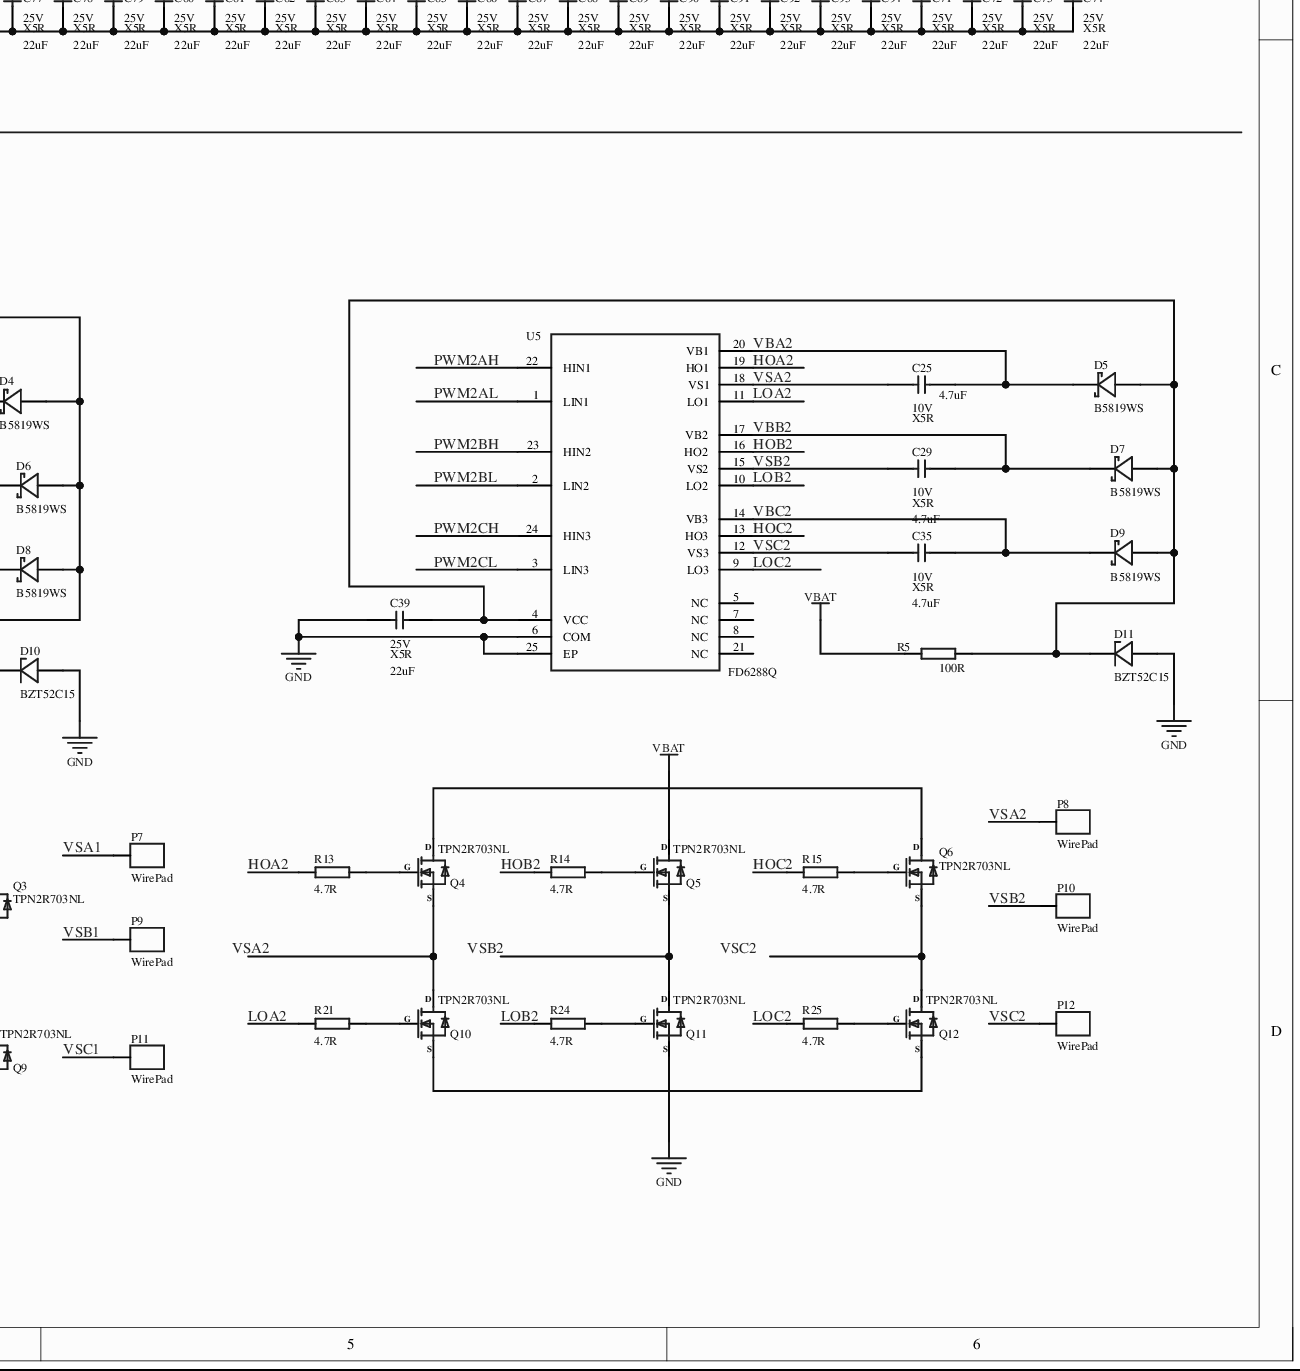
[diagram p0: MISC49862-3.schdoc, bottom right]
# Altium project MISC49862-2.PrjPcb (part 2 of 4)

## Sheet MISC49862-3.schdoc (continued)
### Library data of the parts
C1 = =Value +' '+ Voltage + ' ' + Type: SMD ceramic capacitor; MLCC; 0402(1005);; Device: 4.7uF 10V X5R; Symbol: 4.7uF 0402 10V X5R; Origin Footprint 2: CAPC1005[0402]-L; Origin Footprint 3: CAPC1005[0402]-M; Origin Footprint 4: CAPC1005[0402]-N; Origin Footprint 5: CAPC1005[0402]S-L; Origin Footprint 6: CAPC1005[0402]S-M; UniqueId: b4693cfd16d534cd; AddInBom: yes; Origin Footprint 1: CAPC1005[0402]S-N; Design Item ID: 4.7uF 0402 10V X5R; Library Name: Brushless driver-CYT2BL3-FD6288-FOC-LiteDual; Revision: V1.0; FootprintName: CAPC1005[0402]S-N; ConvertToPcb: yes
C2 = =Value +' '+ Voltage + ' ' + Type: SMD ceramic capacitor; MLCC; 0402(1005);; Device: 100nF 16V X7R; Symbol: 100nF 0402 16V X7R; Origin Footprint 2: CAPC1005[0402]-L; Origin Footprint 3: CAPC1005[0402]-M; Origin Footprint 4: CAPC1005[0402]-N; Origin Footprint 5: CAPC1005[0402]S-L; Origin Footprint 6: CAPC1005[0402]S-M; UniqueId: a2c5d49bc5dde298; AddInBom: yes; Origin Footprint 1: CAPC1005[0402]S-N; Design Item ID: 100nF 0402 16V X7R; Library Name: Brushless driver-CYT2BL3-FD6288-FOC-LiteDual; Revision: V1.0; FootprintName: CAPC1005[0402]S-N; ConvertToPcb: yes
C3 = =Value +' '+ Voltage + ' ' + Type: SMD ceramic capacitor; MLCC; 0402(1005);; Device: 4.7uF 10V X5R; Symbol: 4.7uF 0402 10V X5R; Origin Footprint 2: CAPC1005[0402]-L; Origin Footprint 3: CAPC1005[0402]-M; Origin Footprint 4: CAPC1005[0402]-N; Origin Footprint 5: CAPC1005[0402]S-L; Origin Footprint 6: CAPC1005[0402]S-M; UniqueId: cc82bf2c2e22e605; AddInBom: yes; Origin Footprint 1: CAPC1005[0402]S-N; Design Item ID: 4.7uF 0402 10V X5R; Library Name: Brushless driver-CYT2BL3-FD6288-FOC-LiteDual; Revision: V1.0; FootprintName: CAPC1005[0402]S-N; ConvertToPcb: yes
C4 = =Value +' '+ Voltage + ' ' + Type: SMD ceramic capacitor; MLCC; 0402(1005);; Device: 100nF 16V X7R; Symbol: 100nF 0402 16V X7R; Origin Footprint 2: CAPC1005[0402]-L; Origin Footprint 3: CAPC1005[0402]-M; Origin Footprint 4: CAPC1005[0402]-N; Origin Footprint 5: CAPC1005[0402]S-L; Origin Footprint 6: CAPC1005[0402]S-M; UniqueId: 3a68d3ddabf48558; AddInBom: yes; Origin Footprint 1: CAPC1005[0402]S-N; Design Item ID: 100nF 0402 16V X7R; Library Name: Brushless driver-CYT2BL3-FD6288-FOC-LiteDual; Revision: V1.0; FootprintName: CAPC1005[0402]S-N; ConvertToPcb: yes
C5 = =Value +' '+ Voltage + ' ' + Type: SMD ceramic capacitor; MLCC; 0402(1005);; Device: 2.2uF 10V X5R; Symbol: 2.2uF 0402 10V X5R; Origin Footprint 2: CAPC1005[0402]-L; Origin Footprint 3: CAPC1005[0402]-M; Origin Footprint 4: CAPC1005[0402]-N; Origin Footprint 5: CAPC1005[0402]S-L; Origin Footprint 6: CAPC1005[0402]S-M; UniqueId: ddba3c46cf8b8e66; AddInBom: yes; Origin Footprint 1: CAPC1005[0402]S-N; Design Item ID: 2.2uF 0402 10V X5R; Library Name: Brushless driver-CYT2BL3-FD6288-FOC-LiteDual; Revision: V1.0; FootprintName: CAPC1005[0402]S-N; ConvertToPcb: yes
C6 = =Value +' '+ Voltage + ' ' + Type: SMD ceramic capacitor; MLCC; 0402(1005);; Device: 100nF 16V X7R; Symbol: 100nF 0402 16V X7R; Origin Footprint 2: CAPC1005[0402]-L; Origin Footprint 3: CAPC1005[0402]-M; Origin Footprint 4: CAPC1005[0402]-N; Origin Footprint 5: CAPC1005[0402]S-L; Origin Footprint 6: CAPC1005[0402]S-M; UniqueId: ab4a8fe24fad9fe4; AddInBom: yes; Origin Footprint 1: CAPC1005[0402]S-N; Design Item ID: 100nF 0402 16V X7R; Library Name: Brushless driver-CYT2BL3-FD6288-FOC-LiteDual; Revision: V1.0; FootprintName: CAPC1005[0402]S-N; ConvertToPcb: yes
C7 = =Value +' '+ Voltage + ' ' + Type: SMD ceramic capacitor; MLCC; 0402(1005);; Device: 100nF 16V X7R; Symbol: 100nF 0402 16V X7R; Origin Footprint 2: CAPC1005[0402]-L; Origin Footprint 3: CAPC1005[0402]-M; Origin Footprint 4: CAPC1005[0402]-N; Origin Footprint 5: CAPC1005[0402]S-L; Origin Footprint 6: CAPC1005[0402]S-M; UniqueId: 48d2dd422533522c; AddInBom: yes; Origin Footprint 1: CAPC1005[0402]S-N; Design Item ID: 100nF 0402 16V X7R; Library Name: Brushless driver-CYT2BL3-FD6288-FOC-LiteDual; Revision: V1.0; FootprintName: CAPC1005[0402]S-N; ConvertToPcb: yes
C8 = =Value +' '+ Voltage + ' ' + Type: SMD ceramic capacitor; MLCC; 0402(1005);; Device: 4.7uF 10V X5R; Symbol: 4.7uF 0402 10V X5R; Origin Footprint 2: CAPC1005[0402]-L; Origin Footprint 3: CAPC1005[0402]-M; Origin Footprint 4: CAPC1005[0402]-N; Origin Footprint 5: CAPC1005[0402]S-L; Origin Footprint 6: CAPC1005[0402]S-M; UniqueId: 80f3708378e3d903; AddInBom: yes; Origin Footprint 1: CAPC1005[0402]S-N; Design Item ID: 4.7uF 0402 10V X5R; Library Name: Brushless driver-CYT2BL3-FD6288-FOC-LiteDual; Revision: V1.0; FootprintName: CAPC1005[0402]S-N; ConvertToPcb: yes
C9 = =Value +' '+ Voltage + ' ' + Type: SMD ceramic capacitor; MLCC; 0402(1005);; Device: 4.7uF 10V X5R; Symbol: 4.7uF 0402 10V X5R; Origin Footprint 2: CAPC1005[0402]-L; Origin Footprint 3: CAPC1005[0402]-M; Origin Footprint 4: CAPC1005[0402]-N; Origin Footprint 5: CAPC1005[0402]S-L; Origin Footprint 6: CAPC1005[0402]S-M; UniqueId: 7ddfd2f632a8b17d; AddInBom: yes; Origin Footprint 1: CAPC1005[0402]S-N; Design Item ID: 4.7uF 0402 10V X5R; Library Name: Brushless driver-CYT2BL3-FD6288-FOC-LiteDual; Revision: V1.0; FootprintName: CAPC1005[0402]S-N; ConvertToPcb: yes
C10 = =Value +' '+ Voltage + ' ' + Type: SMD ceramic capacitor; MLCC; 0402(1005);; Device: 100nF 16V X7R; Symbol: 100nF 0402 16V X7R; Origin Footprint 2: CAPC1005[0402]-L; Origin Footprint 3: CAPC1005[0402]-M; Origin Footprint 4: CAPC1005[0402]-N; Origin Footprint 5: CAPC1005[0402]S-L; Origin Footprint 6: CAPC1005[0402]S-M; UniqueId: 3e75135af30e0f04; AddInBom: yes; Origin Footprint 1: CAPC1005[0402]S-N; Design Item ID: 100nF 0402 16V X7R; Library Name: Brushless driver-CYT2BL3-FD6288-FOC-LiteDual; Revision: V1.0; FootprintName: CAPC1005[0402]S-N; ConvertToPcb: yes
C11 = =Value +' '+ Voltage + ' ' + Type: SMD ceramic capacitor; MLCC; 0402(1005);; Device: 100nF 16V X7R; Symbol: 100nF 0402 16V X7R; Origin Footprint 2: CAPC1005[0402]-L; Origin Footprint 3: CAPC1005[0402]-M; Origin Footprint 4: CAPC1005[0402]-N; Origin Footprint 5: CAPC1005[0402]S-L; Origin Footprint 6: CAPC1005[0402]S-M; UniqueId: 20764de07767b3a1; AddInBom: yes; Origin Footprint 1: CAPC1005[0402]S-N; Design Item ID: 100nF 0402 16V X7R; Library Name: Brushless driver-CYT2BL3-FD6288-FOC-LiteDual; Revision: V1.0; FootprintName: CAPC1005[0402]S-N; ConvertToPcb: yes
C12 = =Value +' '+ Voltage + ' ' + Type: SMD ceramic capacitor; MLCC; 0402(1005);; Device: 4.7uF 10V X5R; Symbol: 4.7uF 0402 10V X5R; Origin Footprint 2: CAPC1005[0402]-L; Origin Footprint 3: CAPC1005[0402]-M; Origin Footprint 4: CAPC1005[0402]-N; Origin Footprint 5: CAPC1005[0402]S-L; Origin Footprint 6: CAPC1005[0402]S-M; UniqueId: 26a39bcafcc8ce7c; AddInBom: yes; Origin Footprint 1: CAPC1005[0402]S-N; Design Item ID: 4.7uF 0402 10V X5R; Library Name: Brushless driver-CYT2BL3-FD6288-FOC-LiteDual; Revision: V1.0; FootprintName: CAPC1005[0402]S-N; ConvertToPcb: yes
C13 = =Value +' '+ Voltage + ' ' + Type: SMD ceramic capacitor; MLCC; 0402(1005);; Device: 100nF 16V X7R; Symbol: 100nF 0402 16V X7R; Origin Footprint 2: CAPC1005[0402]-L; Origin Footprint 3: CAPC1005[0402]-M; Origin Footprint 4: CAPC1005[0402]-N; Origin Footprint 5: CAPC1005[0402]S-L; Origin Footprint 6: CAPC1005[0402]S-M; UniqueId: e7ba3aba9f9889c8; AddInBom: yes; Origin Footprint 1: CAPC1005[0402]S-N; Design Item ID: 100nF 0402 16V X7R; Library Name: Brushless driver-CYT2BL3-FD6288-FOC-LiteDual; Revision: V1.0; FootprintName: CAPC1005[0402]S-N; ConvertToPcb: yes
C14 = =Value +' '+ Voltage + ' ' + Type: SMD ceramic capacitor; MLCC; 0402(1005);; Device: 4.7uF 10V X5R; Symbol: 4.7uF 0402 10V X5R; Origin Footprint 2: CAPC1005[0402]-L; Origin Footprint 3: CAPC1005[0402]-M; Origin Footprint 4: CAPC1005[0402]-N; Origin Footprint 5: CAPC1005[0402]S-L; Origin Footprint 6: CAPC1005[0402]S-M; UniqueId: 00361082df9d4549; AddInBom: yes; Origin Footprint 1: CAPC1005[0402]S-N; Design Item ID: 4.7uF 0402 10V X5R; Library Name: Brushless driver-CYT2BL3-FD6288-FOC-LiteDual; Revision: V1.0; FootprintName: CAPC1005[0402]S-N; ConvertToPcb: yes
C15 = =Value +' '+ Voltage + ' ' + Type: SMD ceramic capacitor; MLCC; 0402(1005);; Device: 10pF 50V C0G; Symbol: 10pF 0402 50V C0G; Origin Footprint 2: CAPC1005[0402]-L; Origin Footprint 3: CAPC1005[0402]-M; Origin Footprint 4: CAPC1005[0402]-N; Origin Footprint 5: CAPC1005[0402]S-L; Origin Footprint 6: CAPC1005[0402]S-M; UniqueId: 86bb77bda672094d; AddInBom: yes; Origin Footprint 1: CAPC1005[0402]S-N; Design Item ID: 10pF 0402 50V C0G; Library Name: Brushless driver-CYT2BL3-FD6288-FOC-LiteDual; Revision: V1.0; FootprintName: CAPC1005[0402]S-N; ConvertToPcb: yes
C16 = =Value +' '+ Voltage + ' ' + Type: SMD ceramic capacitor; MLCC; 0402(1005);; Device: 10pF 50V C0G; Symbol: 10pF 0402 50V C0G; Origin Footprint 2: CAPC1005[0402]-L; Origin Footprint 3: CAPC1005[0402]-M; Origin Footprint 4: CAPC1005[0402]-N; Origin Footprint 5: CAPC1005[0402]S-L; Origin Footprint 6: CAPC1005[0402]S-M; UniqueId: c8e923f96b539988; AddInBom: yes; Origin Footprint 1: CAPC1005[0402]S-N; Design Item ID: 10pF 0402 50V C0G; Library Name: Brushless driver-CYT2BL3-FD6288-FOC-LiteDual; Revision: V1.0; FootprintName: CAPC1005[0402]S-N; ConvertToPcb: yes
C17 = =Value +' '+ Voltage + ' ' + Type: SMD ceramic capacitor; MLCC; 0402(1005);; Device: 100nF 16V X7R; Symbol: 100nF 0402 16V X7R; Origin Footprint 2: CAPC1005[0402]-L; Origin Footprint 3: CAPC1005[0402]-M; Origin Footprint 4: CAPC1005[0402]-N; Origin Footprint 5: CAPC1005[0402]S-L; Origin Footprint 6: CAPC1005[0402]S-M; UniqueId: 48700c84863a802e; AddInBom: yes; Origin Footprint 1: CAPC1005[0402]S-N; Design Item ID: 100nF 0402 16V X7R; Library Name: Brushless driver-CYT2BL3-FD6288-FOC-LiteDual; Revision: V1.0; FootprintName: CAPC1005[0402]S-N; ConvertToPcb: yes
C18 = =Value +' '+ Voltage + ' ' + Type: SMD ceramic capacitor; MLCC; 0402(1005);; Device: 4.7uF 10V X5R; Symbol: 4.7uF 0402 10V X5R; Origin Footprint 2: CAPC1005[0402]-L; Origin Footprint 3: CAPC1005[0402]-M; Origin Footprint 4: CAPC1005[0402]-N; Origin Footprint 5: CAPC1005[0402]S-L; Origin Footprint 6: CAPC1005[0402]S-M; UniqueId: d9d0285421fe3ef0; AddInBom: yes; Origin Footprint 1: CAPC1005[0402]S-N; Design Item ID: 4.7uF 0402 10V X5R; Library Name: SEEKFREE_Capacitor; Revision: V1.0; FootprintName: CAPC1005[0402]S-N; ConvertToPcb: yes
C19 = =Value +' '+ Voltage + ' ' + Type: SMD ceramic capacitor; MLCC; 0805(2012);; Device: 22uF 25V X5R; Symbol: 22uF 0805 25V X5R; Origin Footprint 2: CAPC2012[0805]; Origin Footprint 3: CAPC2012[0805]S-L; Origin Footprint 4: CAPC2012[0805]S-M; UniqueId: 9b75bd895f0e39d2; AddInBom: yes; Origin Footprint 1: CAPC2012[0805]S-N; Design Item ID: 22uF 0805 25V X5R; Library Name: SEEKFREE_Capacitor; Revision: V1.0; FootprintName: CAPC2012[0805]S-N; ConvertToPcb: yes
C20 = =Value +' '+ Voltage + ' ' + Type: SMD ceramic capacitor; MLCC; 0805(2012);; Device: 22uF 25V X5R; Symbol: 22uF 0805 25V X5R; Origin Footprint 2: CAPC2012[0805]; Origin Footprint 3: CAPC2012[0805]S-L; Origin Footprint 4: CAPC2012[0805]S-M; UniqueId: 97d7532320e593d5; AddInBom: yes; Origin Footprint 1: CAPC2012[0805]S-N; Design Item ID: 22uF 0805 25V X5R; Library Name: SEEKFREE_Capacitor; Revision: V1.0; FootprintName: CAPC2012[0805]S-N; ConvertToPcb: yes
C21 = =Value +' '+ Voltage + ' ' + Type: SMD ceramic capacitor; MLCC; 0402(1005);; Device: 100nF 16V X7R; Symbol: 100nF 0402 16V X7R; Origin Footprint 2: CAPC1005[0402]-L; Origin Footprint 3: CAPC1005[0402]-M; Origin Footprint 4: CAPC1005[0402]-N; Origin Footprint 5: CAPC1005[0402]S-L; Origin Footprint 6: CAPC1005[0402]S-M; UniqueId: 0259cc883dd91c7a; AddInBom: yes; Origin Footprint 1: CAPC1005[0402]S-N; Design Item ID: 100nF 0402 16V X7R; Library Name: Brushless driver-CYT2BL3-FD6288-FOC-LiteDual; Revision: V1.0; FootprintName: CAPC1005[0402]S-N; ConvertToPcb: yes
C22 = =Value +' '+ Voltage + ' ' + Type: SMD ceramic capacitor; MLCC; 0402(1005);; Device: 220pF 50V X7R; Symbol: 220pF 0402 50V X7R; Origin Footprint 2: CAPC1005[0402]-L; Origin Footprint 3: CAPC1005[0402]-M; Origin Footprint 4: CAPC1005[0402]-N; Origin Footprint 5: CAPC1005[0402]S-L; Origin Footprint 6: CAPC1005[0402]S-M; UniqueId: 7f35450ac3171d20; AddInBom: yes; Origin Footprint 1: CAPC1005[0402]S-N; Design Item ID: 220pF 0402 50V X7R; Library Name: Brushless driver-CYT2BL3-FD6288-FOC-LiteDual; Revision: V1.0; FootprintName: CAPC1005[0402]S-N; ConvertToPcb: yes
C23 = =Value +' '+ Voltage + ' ' + Type: SMD ceramic capacitor; MLCC; 0805(2012);; Device: 22uF 25V X5R; Symbol: 22uF 0805 25V X5R; Origin Footprint 2: CAPC2012[0805]; Origin Footprint 3: CAPC2012[0805]S-L; Origin Footprint 4: CAPC2012[0805]S-M; UniqueId: 8bc5c1e1749a19fa; AddInBom: yes; Origin Footprint 1: CAPC2012[0805]S-N; Design Item ID: 22uF 0805 25V X5R; Library Name: Brushless driver-CYT2BL3-FD6288-FOC-LiteDual; Revision: V1.0; FootprintName: CAPC2012[0805]S-N; ConvertToPcb: yes
C24 = =Value +' '+ Voltage + ' ' + Type: SMD ceramic capacitor; MLCC; 0402(1005);; Device: 100nF 16V X7R; Symbol: 100nF 0402 16V X7R; Origin Footprint 2: CAPC1005[0402]-L; Origin Footprint 3: CAPC1005[0402]-M; Origin Footprint 4: CAPC1005[0402]-N; Origin Footprint 5: CAPC1005[0402]S-L; Origin Footprint 6: CAPC1005[0402]S-M; UniqueId: 7c674fedd66d7165; AddInBom: yes; Origin Footprint 1: CAPC1005[0402]S-N; Design Item ID: 100nF 0402 16V X7R; Library Name: Brushless driver-CYT2BL3-FD6288-FOC-LiteDual; Revision: V1.0; FootprintName: CAPC1005[0402]S-N; ConvertToPcb: yes
C25 = =Value +' '+ Voltage + ' ' + Type: SMD ceramic capacitor; MLCC; 0402(1005);; Device: 4.7uF 10V X5R; Symbol: 4.7uF 0402 10V X5R; Origin Footprint 2: CAPC1005[0402]-L; Origin Footprint 3: CAPC1005[0402]-M; Origin Footprint 4: CAPC1005[0402]-N; Origin Footprint 5: CAPC1005[0402]S-L; Origin Footprint 6: CAPC1005[0402]S-M; UniqueId: d99985aa138ce050; AddInBom: yes; Origin Footprint 1: CAPC1005[0402]S-N; Design Item ID: 4.7uF 0402 10V X5R; Library Name: SEEKFREE_Capacitor; Revision: V1.0; FootprintName: CAPC1005[0402]S-N; ConvertToPcb: yes
C26 = =Value +' '+ Voltage + ' ' + Type: SMD ceramic capacitor; MLCC; 0805(2012);; Device: 22uF 25V X5R; Symbol: 22uF 0805 25V X5R; Origin Footprint 2: CAPC2012[0805]; Origin Footprint 3: CAPC2012[0805]S-L; Origin Footprint 4: CAPC2012[0805]S-M; UniqueId: 5bc8fc857418e778; AddInBom: yes; Origin Footprint 1: CAPC2012[0805]S-N; Design Item ID: 22uF 0805 25V X5R; Library Name: Brushless driver-CYT2BL3-FD6288-FOC-LiteDual; Revision: V1.0; FootprintName: CAPC2012[0805]S-N; ConvertToPcb: yes
C27 = =Value +' '+ Voltage + ' ' + Type: SMD ceramic capacitor; MLCC; 0402(1005);; Device: 100nF 16V X7R; Symbol: 100nF 0402 16V X7R; Origin Footprint 2: CAPC1005[0402]-L; Origin Footprint 3: CAPC1005[0402]-M; Origin Footprint 4: CAPC1005[0402]-N; Origin Footprint 5: CAPC1005[0402]S-L; Origin Footprint 6: CAPC1005[0402]S-M; UniqueId: a26eb100929f0697; AddInBom: yes; Origin Footprint 1: CAPC1005[0402]S-N; Design Item ID: 100nF 0402 16V X7R; Library Name: Brushless driver-CYT2BL3-FD6288-FOC-LiteDual; Revision: V1.0; FootprintName: CAPC1005[0402]S-N; ConvertToPcb: yes
C28 = =Value +' '+ Voltage + ' ' + Type: SMD ceramic capacitor; MLCC; 0402(1005);; Device: 4.7uF 10V X5R; Symbol: 4.7uF 0402 10V X5R; Origin Footprint 2: CAPC1005[0402]-L; Origin Footprint 3: CAPC1005[0402]-M; Origin Footprint 4: CAPC1005[0402]-N; Origin Footprint 5: CAPC1005[0402]S-L; Origin Footprint 6: CAPC1005[0402]S-M; UniqueId: e3aeb17489c0ab5d; AddInBom: yes; Origin Footprint 1: CAPC1005[0402]S-N; Design Item ID: 4.7uF 0402 10V X5R; Library Name: SEEKFREE_Capacitor; Revision: V1.0; FootprintName: CAPC1005[0402]S-N; ConvertToPcb: yes
C29 = =Value +' '+ Voltage + ' ' + Type: SMD ceramic capacitor; MLCC; 0402(1005);; Device: 4.7uF 10V X5R; Symbol: 4.7uF 0402 10V X5R; Origin Footprint 2: CAPC1005[0402]-L; Origin Footprint 3: CAPC1005[0402]-M; Origin Footprint 4: CAPC1005[0402]-N; Origin Footprint 5: CAPC1005[0402]S-L; Origin Footprint 6: CAPC1005[0402]S-M; UniqueId: 5bfcee5f0e3d202c; AddInBom: yes; Origin Footprint 1: CAPC1005[0402]S-N; Design Item ID: 4.7uF 0402 10V X5R; Library Name: SEEKFREE_Capacitor; Revision: V1.0; FootprintName: CAPC1005[0402]S-N; ConvertToPcb: yes
C30 = =Value +' '+ Voltage + ' ' + Type: SMD ceramic capacitor; MLCC; 0402(1005);; Device: 4.7uF 10V X5R; Symbol: 4.7uF 0402 10V X5R; Origin Footprint 2: CAPC1005[0402]-L; Origin Footprint 3: CAPC1005[0402]-M; Origin Footprint 4: CAPC1005[0402]-N; Origin Footprint 5: CAPC1005[0402]S-L; Origin Footprint 6: CAPC1005[0402]S-M; UniqueId: a2ee6ceb65d30336; AddInBom: yes; Origin Footprint 1: CAPC1005[0402]S-N; Design Item ID: 4.7uF 0402 10V X5R; Library Name: SEEKFREE_Capacitor; Revision: V1.0; FootprintName: CAPC1005[0402]S-N; ConvertToPcb: yes
C31 = =Value +' '+ Voltage + ' ' + Type: SMD ceramic capacitor; MLCC; 0402(1005);; Device: 100nF 16V X7R; Symbol: 100nF 0402 16V X7R; Origin Footprint 2: CAPC1005[0402]-L; Origin Footprint 3: CAPC1005[0402]-M; Origin Footprint 4: CAPC1005[0402]-N; Origin Footprint 5: CAPC1005[0402]S-L; Origin Footprint 6: CAPC1005[0402]S-M; UniqueId: cc1d00c51cc12124; AddInBom: yes; Origin Footprint 1: CAPC1005[0402]S-N; Design Item ID: 100nF 0402 16V X7R; Library Name: Brushless driver-CYT2BL3-FD6288-FOC-LiteDual; Revision: V1.0; FootprintName: CAPC1005[0402]S-N; ConvertToPcb: yes
C32 = =Value +' '+ Voltage + ' ' + Type: SMD ceramic capacitor; MLCC; 0402(1005);; Device: 220pF 50V X7R; Symbol: 220pF 0402 50V X7R; Origin Footprint 2: CAPC1005[0402]-L; Origin Footprint 3: CAPC1005[0402]-M; Origin Footprint 4: CAPC1005[0402]-N; Origin Footprint 5: CAPC1005[0402]S-L; Origin Footprint 6: CAPC1005[0402]S-M; UniqueId: d2625f4b4bd439ef; AddInBom: yes; Origin Footprint 1: CAPC1005[0402]S-N; Design Item ID: 220pF 0402 50V X7R; Library Name: Brushless driver-CYT2BL3-FD6288-FOC-LiteDual; Revision: V1.0; FootprintName: CAPC1005[0402]S-N; ConvertToPcb: yes
C33 = =Value +' '+ Voltage + ' ' + Type: SMD ceramic capacitor; MLCC; 0805(2012);; Device: 22uF 25V X5R; Symbol: 22uF 0805 25V X5R; Origin Footprint 2: CAPC2012[0805]; Origin Footprint 3: CAPC2012[0805]S-L; Origin Footprint 4: CAPC2012[0805]S-M; UniqueId: deb55bbe20a101cf; AddInBom: yes; Origin Footprint 1: CAPC2012[0805]S-N; Design Item ID: 22uF 0805 25V X5R; Library Name: Brushless driver-CYT2BL3-FD6288-FOC-LiteDual; Revision: V1.0; FootprintName: CAPC2012[0805]S-N; ConvertToPcb: yes
C34 = =Value +' '+ Voltage + ' ' + Type: SMD ceramic capacitor; MLCC; 0402(1005);; Device: 100nF 16V X7R; Symbol: 100nF 0402 16V X7R; Origin Footprint 2: CAPC1005[0402]-L; Origin Footprint 3: CAPC1005[0402]-M; Origin Footprint 4: CAPC1005[0402]-N; Origin Footprint 5: CAPC1005[0402]S-L; Origin Footprint 6: CAPC1005[0402]S-M; UniqueId: 553def7d7947fca6; AddInBom: yes; Origin Footprint 1: CAPC1005[0402]S-N; Design Item ID: 100nF 0402 16V X7R; Library Name: Brushless driver-CYT2BL3-FD6288-FOC-LiteDual; Revision: V1.0; FootprintName: CAPC1005[0402]S-N; ConvertToPcb: yes
C35 = =Value +' '+ Voltage + ' ' + Type: SMD ceramic capacitor; MLCC; 0402(1005);; Device: 4.7uF 10V X5R; Symbol: 4.7uF 0402 10V X5R; Origin Footprint 2: CAPC1005[0402]-L; Origin Footprint 3: CAPC1005[0402]-M; Origin Footprint 4: CAPC1005[0402]-N; Origin Footprint 5: CAPC1005[0402]S-L; Origin Footprint 6: CAPC1005[0402]S-M; UniqueId: 2b4e6e580c7acde0; AddInBom: yes; Origin Footprint 1: CAPC1005[0402]S-N; Design Item ID: 4.7uF 0402 10V X5R; Library Name: SEEKFREE_Capacitor; Revision: V1.0; FootprintName: CAPC1005[0402]S-N; ConvertToPcb: yes
C36 = =Value +' '+ Voltage + ' ' + Type: SMD ceramic capacitor; MLCC; 0805(2012);; Device: 22uF 25V X5R; Symbol: 22uF 0805 25V X5R; Origin Footprint 2: CAPC2012[0805]; Origin Footprint 3: CAPC2012[0805]S-L; Origin Footprint 4: CAPC2012[0805]S-M; UniqueId: 3db1f6a400993974; AddInBom: yes; Origin Footprint 1: CAPC2012[0805]S-N; Design Item ID: 22uF 0805 25V X5R; Library Name: SEEKFREE_Capacitor; Revision: V1.0; FootprintName: CAPC2012[0805]S-N; ConvertToPcb: yes
C37 = =Value +' '+ Voltage + ' ' + Type: SMD ceramic capacitor; MLCC; 0805(2012);; Device: 22uF 25V X5R; Symbol: 22uF 0805 25V X5R; Origin Footprint 2: CAPC2012[0805]; Origin Footprint 3: CAPC2012[0805]S-L; Origin Footprint 4: CAPC2012[0805]S-M; UniqueId: ff078052695da6b6; AddInBom: yes; Origin Footprint 1: CAPC2012[0805]S-N; Design Item ID: 22uF 0805 25V X5R; Library Name: Brushless driver-CYT2BL3-FD6288-FOC-LiteDual; Revision: V1.0; FootprintName: CAPC2012[0805]S-N; ConvertToPcb: yes
C38 = =Value +' '+ Voltage + ' ' + Type: SMD ceramic capacitor; MLCC; 0402(1005);; Device: 100nF 16V X7R; Symbol: 100nF 0402 16V X7R; Origin Footprint 2: CAPC1005[0402]-L; Origin Footprint 3: CAPC1005[0402]-M; Origin Footprint 4: CAPC1005[0402]-N; Origin Footprint 5: CAPC1005[0402]S-L; Origin Footprint 6: CAPC1005[0402]S-M; UniqueId: 6827ca7a6bd67e26; AddInBom: yes; Origin Footprint 1: CAPC1005[0402]S-N; Design Item ID: 100nF 0402 16V X7R; Library Name: Brushless driver-CYT2BL3-FD6288-FOC-LiteDual; Revision: V1.0; FootprintName: CAPC1005[0402]S-N; ConvertToPcb: yes
C39 = =Value +' '+ Voltage + ' ' + Type: SMD ceramic capacitor; MLCC; 0805(2012);; Device: 22uF 25V X5R; Symbol: 22uF 0805 25V X5R; Origin Footprint 2: CAPC2012[0805]; Origin Footprint 3: CAPC2012[0805]S-L; Origin Footprint 4: CAPC2012[0805]S-M; UniqueId: 54d3d224326b3f8f; AddInBom: yes; Origin Footprint 1: CAPC2012[0805]S-N; Design Item ID: 22uF 0805 25V X5R; Library Name: SEEKFREE_Capacitor; Revision: V1.0; FootprintName: CAPC2012[0805]S-N; ConvertToPcb: yes
C40 = =Value +' '+ Voltage + ' ' + Type: SMD ceramic capacitor; MLCC; 0805(2012);; Device: 22uF 25V X5R; Symbol: 22uF 0805 25V X5R; Origin Footprint 2: CAPC2012[0805]; Origin Footprint 3: CAPC2012[0805]S-L; Origin Footprint 4: CAPC2012[0805]S-M; UniqueId: 12af2948e5a85261; AddInBom: yes; Origin Footprint 1: CAPC2012[0805]S-N; Design Item ID: 22uF 0805 25V X5R; Library Name: SEEKFREE_Capacitor; Revision: V1.0; FootprintName: CAPC2012[0805]S-N; ConvertToPcb: yes
C41 = =Value +' '+ Voltage + ' ' + Type: SMD ceramic capacitor; MLCC; 0805(2012);; Device: 22uF 25V X5R; Symbol: 22uF 0805 25V X5R; Origin Footprint 2: CAPC2012[0805]; Origin Footprint 3: CAPC2012[0805]S-L; Origin Footprint 4: CAPC2012[0805]S-M; UniqueId: c9655d0faea7d93e; AddInBom: yes; Origin Footprint 1: CAPC2012[0805]S-N; Design Item ID: 22uF 0805 25V X5R; Library Name: SEEKFREE_Capacitor; Revision: V1.0; FootprintName: CAPC2012[0805]S-N; ConvertToPcb: yes
C42 = =Value +' '+ Voltage + ' ' + Type: SMD ceramic capacitor; MLCC; 0805(2012);; Device: 22uF 25V X5R; Symbol: 22uF 0805 25V X5R; Origin Footprint 2: CAPC2012[0805]; Origin Footprint 3: CAPC2012[0805]S-L; Origin Footprint 4: CAPC2012[0805]S-M; UniqueId: d39ee3bf0fadc3c1; AddInBom: yes; Origin Footprint 1: CAPC2012[0805]S-N; Design Item ID: 22uF 0805 25V X5R; Library Name: SEEKFREE_Capacitor; Revision: V1.0; FootprintName: CAPC2012[0805]S-N; ConvertToPcb: yes
C43 = =Value +' '+ Voltage + ' ' + Type: SMD ceramic capacitor; MLCC; 0805(2012);; Device: 22uF 25V X5R; Symbol: 22uF 0805 25V X5R; Origin Footprint 2: CAPC2012[0805]; Origin Footprint 3: CAPC2012[0805]S-L; Origin Footprint 4: CAPC2012[0805]S-M; UniqueId: ad7e9e1612356ddb; AddInBom: yes; Origin Footprint 1: CAPC2012[0805]S-N; Design Item ID: 22uF 0805 25V X5R; Library Name: SEEKFREE_Capacitor; Revision: V1.0; FootprintName: CAPC2012[0805]S-N; ConvertToPcb: yes
C44 = =Value +' '+ Voltage + ' ' + Type: SMD ceramic capacitor; MLCC; 0805(2012);; Device: 22uF 25V X5R; Symbol: 22uF 0805 25V X5R; Origin Footprint 2: CAPC2012[0805]; Origin Footprint 3: CAPC2012[0805]S-L; Origin Footprint 4: CAPC2012[0805]S-M; UniqueId: 49133e3f49d3504d; AddInBom: yes; Origin Footprint 1: CAPC2012[0805]S-N; Design Item ID: 22uF 0805 25V X5R; Library Name: SEEKFREE_Capacitor; Revision: V1.0; FootprintName: CAPC2012[0805]S-N; ConvertToPcb: yes
C45 = =Value +' '+ Voltage + ' ' + Type: SMD ceramic capacitor; MLCC; 0805(2012);; Device: 22uF 25V X5R; Symbol: 22uF 0805 25V X5R; Origin Footprint 2: CAPC2012[0805]; Origin Footprint 3: CAPC2012[0805]S-L; Origin Footprint 4: CAPC2012[0805]S-M; UniqueId: 9dabde1b2911a551; AddInBom: yes; Origin Footprint 1: CAPC2012[0805]S-N; Design Item ID: 22uF 0805 25V X5R; Library Name: SEEKFREE_Capacitor; Revision: V1.0; FootprintName: CAPC2012[0805]S-N; ConvertToPcb: yes
C46 = =Value +' '+ Voltage + ' ' + Type: SMD ceramic capacitor; MLCC; 0805(2012);; Device: 22uF 25V X5R; Symbol: 22uF 0805 25V X5R; Origin Footprint 2: CAPC2012[0805]; Origin Footprint 3: CAPC2012[0805]S-L; Origin Footprint 4: CAPC2012[0805]S-M; UniqueId: df918f74c5ced612; AddInBom: yes; Origin Footprint 1: CAPC2012[0805]S-N; Design Item ID: 22uF 0805 25V X5R; Library Name: SEEKFREE_Capacitor; Revision: V1.0; FootprintName: CAPC2012[0805]S-N; ConvertToPcb: yes
C47 = =Value +' '+ Voltage + ' ' + Type: SMD ceramic capacitor; MLCC; 0805(2012);; Device: 22uF 25V X5R; Symbol: 22uF 0805 25V X5R; Origin Footprint 2: CAPC2012[0805]; Origin Footprint 3: CAPC2012[0805]S-L; Origin Footprint 4: CAPC2012[0805]S-M; UniqueId: 64621f1995cfd5bc; AddInBom: yes; Origin Footprint 1: CAPC2012[0805]S-N; Design Item ID: 22uF 0805 25V X5R; Library Name: SEEKFREE_Capacitor; Revision: V1.0; FootprintName: CAPC2012[0805]S-N; ConvertToPcb: yes
C48 = =Value +' '+ Voltage + ' ' + Type: SMD ceramic capacitor; MLCC; 0805(2012);; Device: 22uF 25V X5R; Symbol: 22uF 0805 25V X5R; Origin Footprint 2: CAPC2012[0805]; Origin Footprint 3: CAPC2012[0805]S-L; Origin Footprint 4: CAPC2012[0805]S-M; UniqueId: 808ebf677d8d6d64; AddInBom: yes; Origin Footprint 1: CAPC2012[0805]S-N; Design Item ID: 22uF 0805 25V X5R; Library Name: SEEKFREE_Capacitor; Revision: V1.0; FootprintName: CAPC2012[0805]S-N; ConvertToPcb: yes
C49 = =Value +' '+ Voltage + ' ' + Type: SMD ceramic capacitor; MLCC; 0402(1005);; Device: 100nF 16V X7R; Symbol: 100nF 0402 16V X7R; Origin Footprint 2: CAPC1005[0402]-L; Origin Footprint 3: CAPC1005[0402]-M; Origin Footprint 4: CAPC1005[0402]-N; Origin Footprint 5: CAPC1005[0402]S-L; Origin Footprint 6: CAPC1005[0402]S-M; UniqueId: 91fd74edebd22ea1; AddInBom: yes; Origin Footprint 1: CAPC1005[0402]S-N; Design Item ID: 100nF 0402 16V X7R; Library Name: Brushless driver-CYT2BL3-FD6288-FOC-LiteDual; Revision: V1.0; FootprintName: CAPC1005[0402]S-N; ConvertToPcb: yes
C50 = =Value +' '+ Voltage + ' ' + Type: SMD ceramic capacitor; MLCC; 0805(2012);; Device: 22uF 25V X5R; Symbol: 22uF 0805 25V X5R; Origin Footprint 2: CAPC2012[0805]; Origin Footprint 3: CAPC2012[0805]S-L; Origin Footprint 4: CAPC2012[0805]S-M; UniqueId: 32f6df7045cd6eaa; AddInBom: yes; Origin Footprint 1: CAPC2012[0805]S-N; Design Item ID: 22uF 0805 25V X5R; Library Name: SEEKFREE_Capacitor; Revision: V1.0; FootprintName: CAPC2012[0805]S-N; ConvertToPcb: yes
C51 = =Value +' '+ Voltage + ' ' + Type: SMD ceramic capacitor; MLCC; 0805(2012);; Device: 22uF 25V X5R; Symbol: 22uF 0805 25V X5R; Origin Footprint 2: CAPC2012[0805]; Origin Footprint 3: CAPC2012[0805]S-L; Origin Footprint 4: CAPC2012[0805]S-M; UniqueId: d35436b77a732af0; AddInBom: yes; Origin Footprint 1: CAPC2012[0805]S-N; Design Item ID: 22uF 0805 25V X5R; Library Name: SEEKFREE_Capacitor; Revision: V1.0; FootprintName: CAPC2012[0805]S-N; ConvertToPcb: yes
C52 = =Value +' '+ Voltage + ' ' + Type: SMD ceramic capacitor; MLCC; 0805(2012);; Device: 22uF 25V X5R; Symbol: 22uF 0805 25V X5R; Origin Footprint 2: CAPC2012[0805]; Origin Footprint 3: CAPC2012[0805]S-L; Origin Footprint 4: CAPC2012[0805]S-M; UniqueId: 35d858017be1d91e; AddInBom: yes; Origin Footprint 1: CAPC2012[0805]S-N; Design Item ID: 22uF 0805 25V X5R; Library Name: SEEKFREE_Capacitor; Revision: V1.0; FootprintName: CAPC2012[0805]S-N; ConvertToPcb: yes
C53 = =Value +' '+ Voltage + ' ' + Type: SMD ceramic capacitor; MLCC; 0805(2012);; Device: 22uF 25V X5R; Symbol: 22uF 0805 25V X5R; Origin Footprint 2: CAPC2012[0805]; Origin Footprint 3: CAPC2012[0805]S-L; Origin Footprint 4: CAPC2012[0805]S-M; UniqueId: af7046427a4bfdfb; AddInBom: yes; Origin Footprint 1: CAPC2012[0805]S-N; Design Item ID: 22uF 0805 25V X5R; Library Name: SEEKFREE_Capacitor; Revision: V1.0; FootprintName: CAPC2012[0805]S-N; ConvertToPcb: yes
C54 = =Value +' '+ Voltage + ' ' + Type: SMD ceramic capacitor; MLCC; 0805(2012);; Device: 22uF 25V X5R; Symbol: 22uF 0805 25V X5R; Origin Footprint 2: CAPC2012[0805]; Origin Footprint 3: CAPC2012[0805]S-L; Origin Footprint 4: CAPC2012[0805]S-M; UniqueId: 65328433fb04ddb7; AddInBom: yes; Origin Footprint 1: CAPC2012[0805]S-N; Design Item ID: 22uF 0805 25V X5R; Library Name: SEEKFREE_Capacitor; Revision: V1.0; FootprintName: CAPC2012[0805]S-N; ConvertToPcb: yes
C55 = =Value +' '+ Voltage + ' ' + Type: SMD ceramic capacitor; MLCC; 0805(2012);; Device: 22uF 25V X5R; Symbol: 22uF 0805 25V X5R; Origin Footprint 2: CAPC2012[0805]; Origin Footprint 3: CAPC2012[0805]S-L; Origin Footprint 4: CAPC2012[0805]S-M; UniqueId: 82ba1af55b3917e5; AddInBom: yes; Origin Footprint 1: CAPC2012[0805]S-N; Design Item ID: 22uF 0805 25V X5R; Library Name: SEEKFREE_Capacitor; Revision: V1.0; FootprintName: CAPC2012[0805]S-N; ConvertToPcb: yes
C56 = =Value +' '+ Voltage + ' ' + Type: SMD ceramic capacitor; MLCC; 0805(2012);; Device: 22uF 25V X5R; Symbol: 22uF 0805 25V X5R; Origin Footprint 2: CAPC2012[0805]; Origin Footprint 3: CAPC2012[0805]S-L; Origin Footprint 4: CAPC2012[0805]S-M; UniqueId: a22d741cda083e99; AddInBom: yes; Origin Footprint 1: CAPC2012[0805]S-N; Design Item ID: 22uF 0805 25V X5R; Library Name: SEEKFREE_Capacitor; Revision: V1.0; FootprintName: CAPC2012[0805]S-N; ConvertToPcb: yes
C57 = =Value +' '+ Voltage + ' ' + Type: SMD ceramic capacitor; MLCC; 0805(2012);; Device: 22uF 25V X5R; Symbol: 22uF 0805 25V X5R; Origin Footprint 2: CAPC2012[0805]; Origin Footprint 3: CAPC2012[0805]S-L; Origin Footprint 4: CAPC2012[0805]S-M; UniqueId: 21dd5459dde3f81c; AddInBom: yes; Origin Footprint 1: CAPC2012[0805]S-N; Design Item ID: 22uF 0805 25V X5R; Library Name: SEEKFREE_Capacitor; Revision: V1.0; FootprintName: CAPC2012[0805]S-N; ConvertToPcb: yes
C58 = =Value +' '+ Voltage + ' ' + Type: SMD ceramic capacitor; MLCC; 0805(2012);; Device: 22uF 25V X5R; Symbol: 22uF 0805 25V X5R; Origin Footprint 2: CAPC2012[0805]; Origin Footprint 3: CAPC2012[0805]S-L; Origin Footprint 4: CAPC2012[0805]S-M; UniqueId: 6c1fb86984bf7302; AddInBom: yes; Origin Footprint 1: CAPC2012[0805]S-N; Design Item ID: 22uF 0805 25V X5R; Library Name: SEEKFREE_Capacitor; Revision: V1.0; FootprintName: CAPC2012[0805]S-N; ConvertToPcb: yes
C59 = =Value +' '+ Voltage + ' ' + Type: SMD ceramic capacitor; MLCC; 0805(2012);; Device: 22uF 25V X5R; Symbol: 22uF 0805 25V X5R; Origin Footprint 2: CAPC2012[0805]; Origin Footprint 3: CAPC2012[0805]S-L; Origin Footprint 4: CAPC2012[0805]S-M; UniqueId: 9b91e7356bb9865f; AddInBom: yes; Origin Footprint 1: CAPC2012[0805]S-N; Design Item ID: 22uF 0805 25V X5R; Library Name: SEEKFREE_Capacitor; Revision: V1.0; FootprintName: CAPC2012[0805]S-N; ConvertToPcb: yes
C60 = =Value +' '+ Voltage + ' ' + Type: SMD ceramic capacitor; MLCC; 0805(2012);; Device: 22uF 25V X5R; Symbol: 22uF 0805 25V X5R; Origin Footprint 2: CAPC2012[0805]; Origin Footprint 3: CAPC2012[0805]S-L; Origin Footprint 4: CAPC2012[0805]S-M; UniqueId: 769677d4f8f56233; AddInBom: yes; Origin Footprint 1: CAPC2012[0805]S-N; Design Item ID: 22uF 0805 25V X5R; Library Name: SEEKFREE_Capacitor; Revision: V1.0; FootprintName: CAPC2012[0805]S-N; ConvertToPcb: yes
C61 = =Value +' '+ Voltage + ' ' + Type: SMD ceramic capacitor; MLCC; 0805(2012);; Device: 22uF 25V X5R; Symbol: 22uF 0805 25V X5R; Origin Footprint 2: CAPC2012[0805]; Origin Footprint 3: CAPC2012[0805]S-L; Origin Footprint 4: CAPC2012[0805]S-M; UniqueId: 3745dda5a27601a3; AddInBom: yes; Origin Footprint 1: CAPC2012[0805]S-N; Design Item ID: 22uF 0805 25V X5R; Library Name: SEEKFREE_Capacitor; Revision: V1.0; FootprintName: CAPC2012[0805]S-N; ConvertToPcb: yes
C62 = =Value +' '+ Voltage + ' ' + Type: SMD ceramic capacitor; MLCC; 0805(2012);; Device: 22uF 25V X5R; Symbol: 22uF 0805 25V X5R; Origin Footprint 2: CAPC2012[0805]; Origin Footprint 3: CAPC2012[0805]S-L; Origin Footprint 4: CAPC2012[0805]S-M; UniqueId: 4b556904310d1556; AddInBom: yes; Origin Footprint 1: CAPC2012[0805]S-N; Design Item ID: 22uF 0805 25V X5R; Library Name: SEEKFREE_Capacitor; Revision: V1.0; FootprintName: CAPC2012[0805]S-N; ConvertToPcb: yes
C63 = =Value +' '+ Voltage + ' ' + Type: SMD ceramic capacitor; MLCC; 0805(2012);; Device: 22uF 25V X5R; Symbol: 22uF 0805 25V X5R; Origin Footprint 2: CAPC2012[0805]; Origin Footprint 3: CAPC2012[0805]S-L; Origin Footprint 4: CAPC2012[0805]S-M; UniqueId: b3cb865a57c4a975; AddInBom: yes; Origin Footprint 1: CAPC2012[0805]S-N; Design Item ID: 22uF 0805 25V X5R; Library Name: SEEKFREE_Capacitor; Revision: V1.0; FootprintName: CAPC2012[0805]S-N; ConvertToPcb: yes
C64 = =Value +' '+ Voltage + ' ' + Type: SMD ceramic capacitor; MLCC; 0805(2012);; Device: 22uF 25V X5R; Symbol: 22uF 0805 25V X5R; Origin Footprint 2: CAPC2012[0805]; Origin Footprint 3: CAPC2012[0805]S-L; Origin Footprint 4: CAPC2012[0805]S-M; UniqueId: 9944326385f1aa7b; AddInBom: yes; Origin Footprint 1: CAPC2012[0805]S-N; Design Item ID: 22uF 0805 25V X5R; Library Name: SEEKFREE_Capacitor; Revision: V1.0; FootprintName: CAPC2012[0805]S-N; ConvertToPcb: yes
C65 = =Value +' '+ Voltage + ' ' + Type: SMD ceramic capacitor; MLCC; 0805(2012);; Device: 22uF 25V X5R; Symbol: 22uF 0805 25V X5R; Origin Footprint 2: CAPC2012[0805]; Origin Footprint 3: CAPC2012[0805]S-L; Origin Footprint 4: CAPC2012[0805]S-M; UniqueId: ac9f836745bfd3f0; AddInBom: yes; Origin Footprint 1: CAPC2012[0805]S-N; Design Item ID: 22uF 0805 25V X5R; Library Name: SEEKFREE_Capacitor; Revision: V1.0; FootprintName: CAPC2012[0805]S-N; ConvertToPcb: yes
C66 = =Value +' '+ Voltage + ' ' + Type: SMD ceramic capacitor; MLCC; 0805(2012);; Device: 22uF 25V X5R; Symbol: 22uF 0805 25V X5R; Origin Footprint 2: CAPC2012[0805]; Origin Footprint 3: CAPC2012[0805]S-L; Origin Footprint 4: CAPC2012[0805]S-M; UniqueId: fb27f7370dbf7a2e; AddInBom: yes; Origin Footprint 1: CAPC2012[0805]S-N; Design Item ID: 22uF 0805 25V X5R; Library Name: SEEKFREE_Capacitor; Revision: V1.0; FootprintName: CAPC2012[0805]S-N; ConvertToPcb: yes
C67 = =Value +' '+ Voltage + ' ' + Type: SMD ceramic capacitor; MLCC; 0805(2012);; Device: 22uF 25V X5R; Symbol: 22uF 0805 25V X5R; Origin Footprint 2: CAPC2012[0805]; Origin Footprint 3: CAPC2012[0805]S-L; Origin Footprint 4: CAPC2012[0805]S-M; UniqueId: 790facc1dd52bc03; AddInBom: yes; Origin Footprint 1: CAPC2012[0805]S-N; Design Item ID: 22uF 0805 25V X5R; Library Name: SEEKFREE_Capacitor; Revision: V1.0; FootprintName: CAPC2012[0805]S-N; ConvertToPcb: yes
C68 = =Value +' '+ Voltage + ' ' + Type: SMD ceramic capacitor; MLCC; 0805(2012);; Device: 22uF 25V X5R; Symbol: 22uF 0805 25V X5R; Origin Footprint 2: CAPC2012[0805]; Origin Footprint 3: CAPC2012[0805]S-L; Origin Footprint 4: CAPC2012[0805]S-M; UniqueId: 695de859447a278b; AddInBom: yes; Origin Footprint 1: CAPC2012[0805]S-N; Design Item ID: 22uF 0805 25V X5R; Library Name: SEEKFREE_Capacitor; Revision: V1.0; FootprintName: CAPC2012[0805]S-N; ConvertToPcb: yes
C69 = =Value +' '+ Voltage + ' ' + Type: SMD ceramic capacitor; MLCC; 0805(2012);; Device: 22uF 25V X5R; Symbol: 22uF 0805 25V X5R; Origin Footprint 2: CAPC2012[0805]; Origin Footprint 3: CAPC2012[0805]S-L; Origin Footprint 4: CAPC2012[0805]S-M; UniqueId: ed5e3f159d100c7c; AddInBom: yes; Origin Footprint 1: CAPC2012[0805]S-N; Design Item ID: 22uF 0805 25V X5R; Library Name: SEEKFREE_Capacitor; Revision: V1.0; FootprintName: CAPC2012[0805]S-N; ConvertToPcb: yes
C70 = =Value +' '+ Voltage + ' ' + Type: SMD ceramic capacitor; MLCC; 0805(2012);; Device: 22uF 25V X5R; Symbol: 22uF 0805 25V X5R; Origin Footprint 2: CAPC2012[0805]; Origin Footprint 3: CAPC2012[0805]S-L; Origin Footprint 4: CAPC2012[0805]S-M; UniqueId: ef22f62b38d240f9; AddInBom: yes; Origin Footprint 1: CAPC2012[0805]S-N; Design Item ID: 22uF 0805 25V X5R; Library Name: SEEKFREE_Capacitor; Revision: V1.0; FootprintName: CAPC2012[0805]S-N; ConvertToPcb: yes